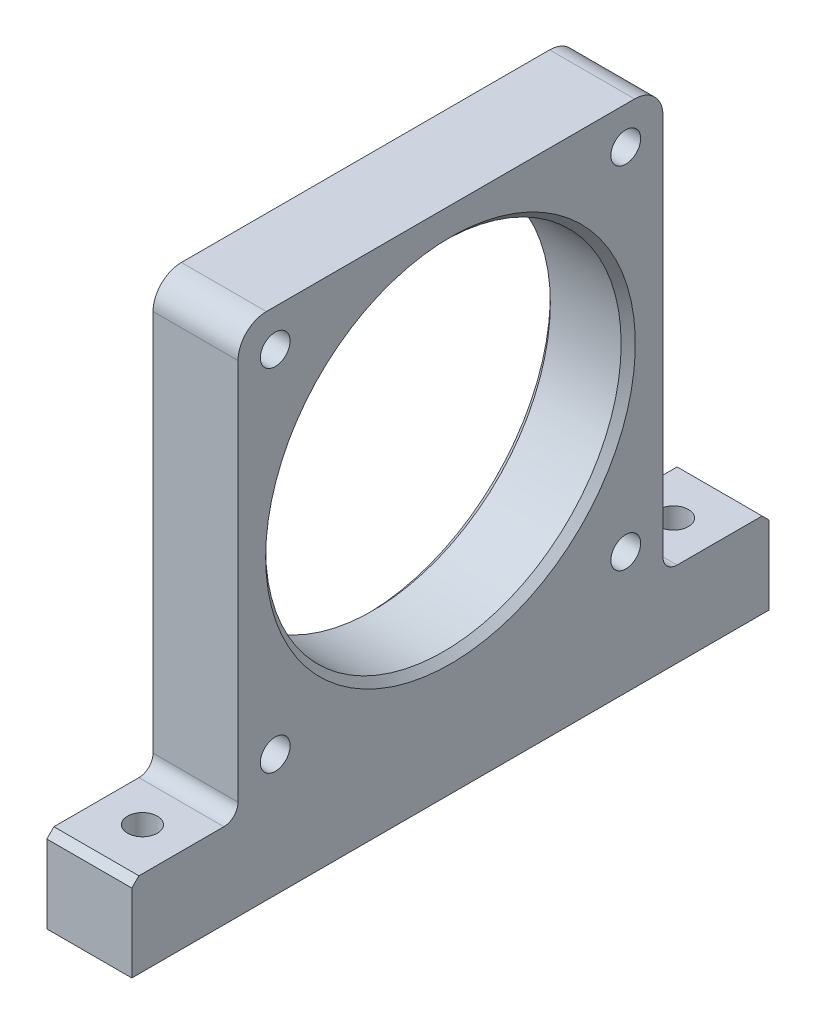
from build123d import *

# Parameters (mm, degrees)
SKETCH1_R             = 25.1
BOSS_EXTRUDE1_DEPTH   = 6
FILLET1_R             = 4
FILLET2_R             = 2
CHAMFER1_SIZE         = 1
M5_TAPPED_HOLE2_D     = 4.2
M5_TAPPED_HOLE1_D     = 4.2
M5_TAPPED_HOLE1_DEPTH = 14
M5_TAPPED_HOLE1_TIP   = 1.2618073
CHAMFER2_SIZE         = 1


with BuildPart() as part:
    # Sketch1 → Boss-Extrude1 (new, symmetric)
    with BuildSketch(Plane(origin=(0, 0, 0), x_dir=(0, 0, -1), z_dir=(1, 0, 0))):
        Polygon((-45, 0), (45, 0), (45, 12), (30, 12), (30, 72), (-30, 72), (-30, 12), (-45, 12), align=None)
        with Locations((0, 42)):
            Circle(SKETCH1_R, mode=Mode.SUBTRACT)
    extrude(amount=BOSS_EXTRUDE1_DEPTH, both=True)

    # Fillet1
    fillet1_edges = [part.edges().sort_by_distance(p)[0] for p in [
        (0, 72, 30),
        (0, 72, -30),
    ]]
    fillet(fillet1_edges, radius=FILLET1_R)

    # Fillet2
    fillet2_edges = [part.edges().sort_by_distance(p)[0] for p in [
        (0, 12, 30),
        (0, 12, -30),
    ]]
    fillet(fillet2_edges, radius=FILLET2_R)

    # Chamfer1
    chamfer1_edges = [part.edges().sort_by_distance(p)[0] for p in [
        (0, 12, 45),
        (0, 12, -45),
    ]]
    chamfer(chamfer1_edges, length=CHAMFER1_SIZE)

    # M5 Tapped Hole2 (through all)
    with Locations(Plane(origin=(0, 12, 0), x_dir=(1, 0, 0), z_dir=(0, 1, 0))):
        with Locations((0, -37.5), (0, 37.5)):
            Hole(M5_TAPPED_HOLE2_D / 2)

    # M5 Tapped Hole1
    with Locations(Plane(origin=(6, 0, 0), x_dir=(0, 0, -1), z_dir=(1, 0, 0))):
        with Locations((-24.748737342, 66.748737342), (24.748737342, 66.748737342), (24.748737342, 17.251262658), (-24.748737342, 17.251262658)):
            Hole(M5_TAPPED_HOLE1_D / 2, depth=M5_TAPPED_HOLE1_DEPTH)
            with Locations((0, 0, -(M5_TAPPED_HOLE1_DEPTH + M5_TAPPED_HOLE1_TIP / 2))):  # 118° drill point
                Cone(0, M5_TAPPED_HOLE1_D / 2, M5_TAPPED_HOLE1_TIP, mode=Mode.SUBTRACT)

    # Chamfer2
    chamfer2_edges = [part.edges().sort_by_distance(p)[0] for p in [
        (-6, 42, 25.1),
        (6, 42, 25.1),
    ]]
    chamfer(chamfer2_edges, length=CHAMFER2_SIZE)


solid = part.part
